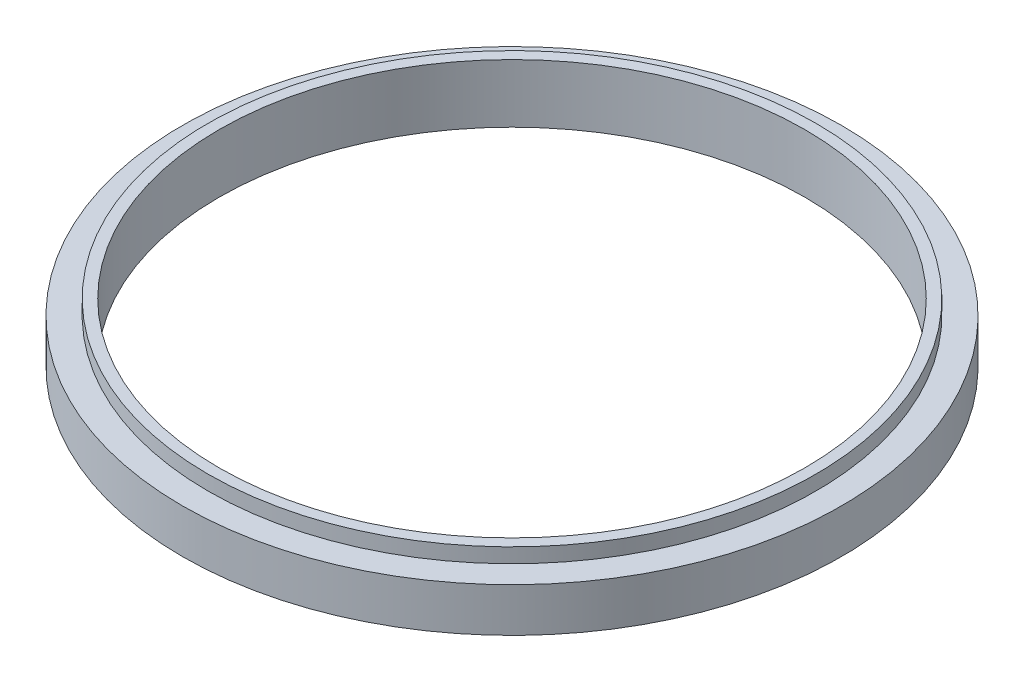
SolidWorks part; units mm, degrees
ref_plane "Front Plane" through (0, 0, 0) normal (0, 0, 1) x (1, 0, 0)
ref_plane "Top Plane" through (0, 0, 0) normal (0, 1, 0) x (1, 0, 0)
ref_plane "Right Plane" through (0, 0, 0) normal (1, 0, 0) x (0, 0, -1)
sketch "Sketch1" plane through (0, 0, 0) normal (0, 1, 0) x (1, 0, 0)
  circle A0 centre (0, 0) radius 45
  circle A1 centre (0, 0) radius 40
  dimension "D1" = 80
  dimension "D2" = 90
extrude "Boss-Extrude1" add sketch "Sketch1" along normal blind 6
sketch "Sketch2" plane through (0, 6, 0) normal (0, 1, 0) x (1, 0, 0)
  circle A0 centre (0, 0) radius 40
  circle A1 centre (0, 0) radius 41.5
  dimension "D1" = 80
  dimension "D2" = 83
extrude "Boss-Extrude2" add sketch "Sketch2" along normal blind 2
